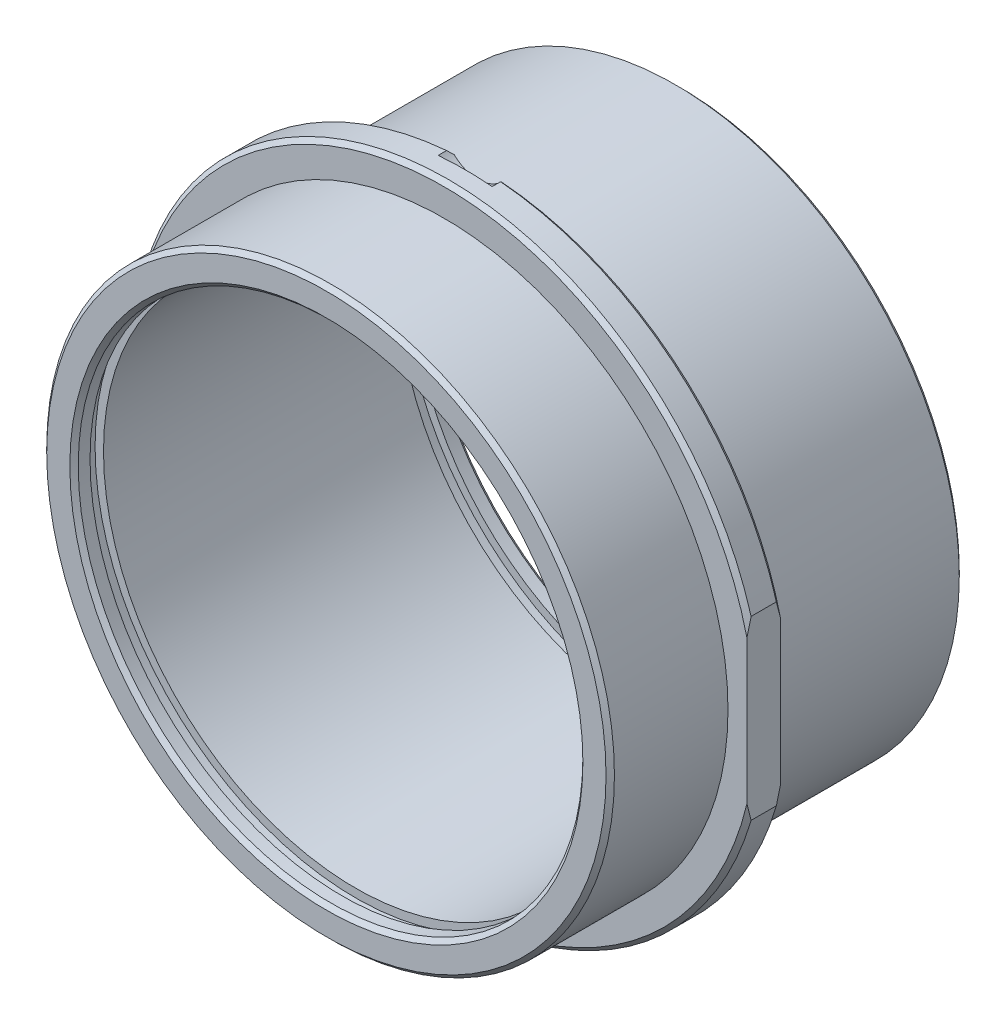
SolidWorks part; units mm, degrees
material "P20"
ref_plane "Front Plane" through (0, 0, 0) normal (0, 0, 1) x (1, 0, 0)
ref_plane "Top Plane" through (0, 0, 0) normal (0, 1, 0) x (1, 0, 0)
ref_plane "Right Plane" through (0, 0, 0) normal (1, 0, 0) x (0, 0, -1)
sketch "Sketch1" plane through (0, 0, 0) normal (0, 0, 1) x (1, 0, 0)
  circle A1 centre (0, 0) radius 75
  dimension "D2" = 150
extrude "Boss-Extrude1" add sketch "Sketch1" along normal blind 8
sketch "Sketch2" plane through (0, 0, 8) normal (0, 0, 1) x (1, 0, 0)
  circle A0 centre (0, 0) radius 67.5
  dimension "D1" = 135
extrude "Boss-Extrude2" add sketch "Sketch2" along normal blind 28 and the other way blind 56
sketch "Sketch3" plane through (0, 0, 36) normal (0, 0, 1) x (1, 0, 0)
  circle A0 centre (0, 0) radius 60
  dimension "D1" = 120
extrude "Cut-Extrude1" cut sketch "Sketch3" against normal blind 160
sketch "Sketch4" plane through (0, 0, 0) normal (0, 1, 0) x (1, 0, 0)
  line L0 (0, 49.9905) -> (0, -131.7913) construction
  line L2 (-56.8023, -29) -> (-62, -29)
  line L3 (-56.8023, -29) -> (-56.8023, -32.2)
  line L4 (-56.8023, -32.2) -> (-62, -32.2)
  line L5 (-62, -29) -> (-62, -32.2)
  line L6 (-67.5, -36) -> (67.5, -36) construction
  line L9 (-62, 44.2) -> (-56.8023, 44.2)
  line L10 (-62, 44.2) -> (-62, 41)
  line L11 (-62, 41) -> (-56.8023, 41)
  line L12 (-56.8023, 44.2) -> (-56.8023, 41)
  dimension "D1" = 3.2
  dimension "D2" = 7
  dimension "D3" = 62
  dimension "D4" = 3.2
  dimension "D5" = 70
revolve "Cut-Revolve1" cut sketch "Sketch4" angle 360 about L0
chamfer "Chamfer1" distance 1 angle 45 6 edges at (67.5, 0, 36) (75, 0, 0) (75, 0, 8) (60, 0, 36) (67.5, 0, -48) (60, 0, -48)
sketch "Sketch5" plane through (0, 0, 0) normal (0, 0, -1) x (-1, 0, 0)
  line L0 (0, 173.1483) -> (0, -190.9667) construction
  line L1 (0, 0) -> (-225.6766, 0) construction
  line L2 (-132, 75) -> (-72, 75)
  line L3 (-132, 75) -> (-132, -75)
  line L4 (-132, -75) -> (-72, -75)
  line L5 (-72, 75) -> (-72, -75)
  line L6 (132, 75) -> (72, 75)
  line L7 (132, 75) -> (132, -75)
  line L8 (132, -75) -> (72, -75)
  line L9 (72, 75) -> (72, -75)
  dimension "D1" = 60
  dimension "D2" = 60
  dimension "D3" = 150
  dimension "D4" = 144
extrude "Cut-Extrude2" cut sketch "Sketch5" against normal blind 72
sketch "Sketch6" plane through (0, 0, 0) normal (0, 0, 1) x (1, 0, 0)
  line L0 (-153.78, 0) -> (143.4738, 0) construction
  line L1 (0, 79.5) -> (0, -79.5) construction
  circle A0 centre (0, 79.5) radius 8
  circle A1 centre (0, -79.5) radius 8
  circle A2 centre (0, 0) radius 79.5 construction
  dimension "D1" = 16
  dimension "D2" = 159
extrude "Cut-Extrude3" cut sketch "Sketch6" along normal blind 3
